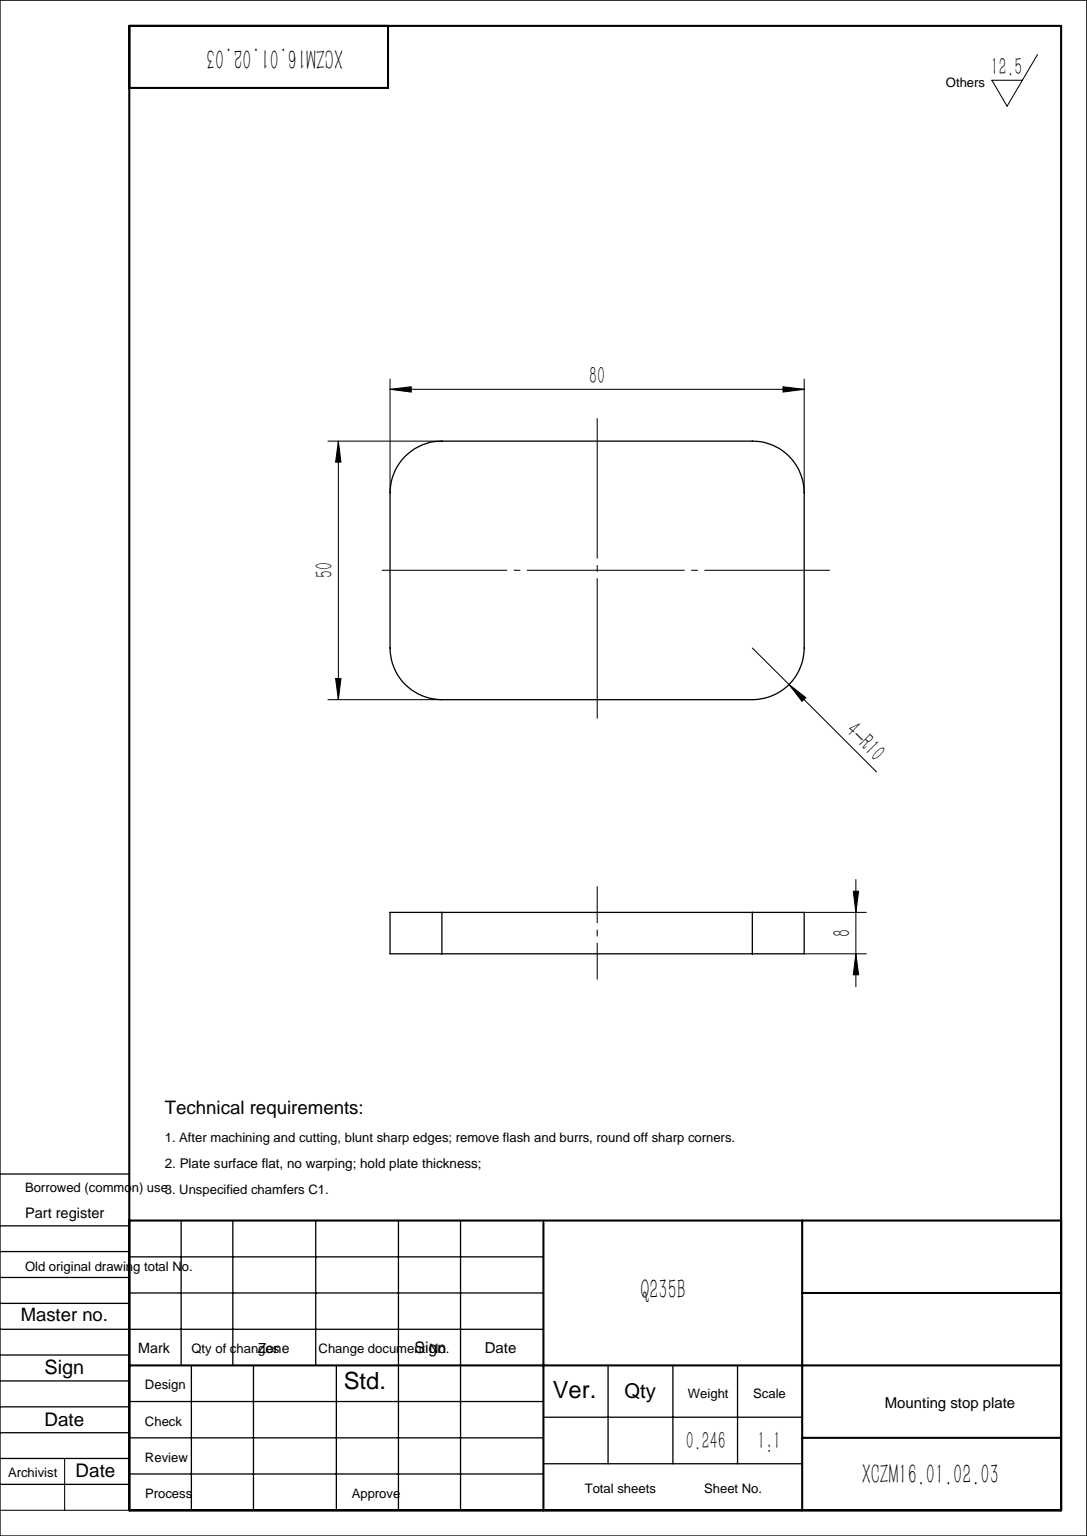
SolidWorks part; units mm, degrees
material "Q235B"
ref_plane "Front Plane" through (0, 0, 0) normal (0, 0, 1) x (1, 0, 0)
ref_plane "Top Plane" through (0, 0, 0) normal (0, 1, 0) x (1, 0, 0)
ref_plane "Right Plane" through (0, 0, 0) normal (1, 0, 0) x (0, 0, -1)
sketch "Sketch1" plane through (0, 0, 0) normal (0, 0, 1) x (1, 0, 0)
  line L1 (30, -25) -> (-30, -25)
  line L2 (40, -15) -> (40, 15)
  line L3 (30, 25) -> (-30, 25)
  line L4 (-40, -15) -> (-40, 15)
  line L5 (40, -25) -> (-40, 25) construction
  line L6 (40, 25) -> (-40, -25) construction
  arc A0 (-30, -25) -> (-40, -15) centre (-30, -15) cw
  arc A1 (40, 15) -> (30, 25) centre (30, 15) ccw
  arc A2 (30, -25) -> (40, -15) centre (30, -15) ccw
  arc A3 (-30, 25) -> (-40, 15) centre (-30, 15) ccw
  point P0 (0, 0)
  dimension "D3" = 10
  dimension "D1" = 50
  dimension "D2" = 80
extrude "Boss-Extrude1" add sketch "Sketch1" along normal blind 8
